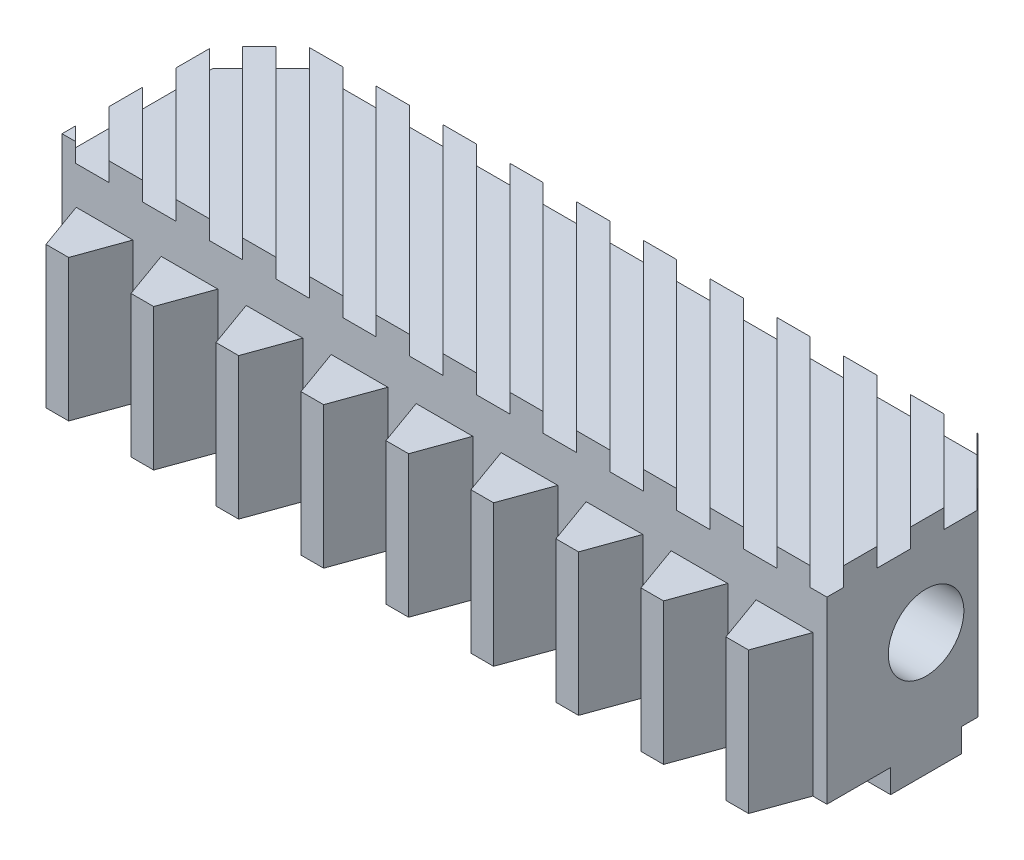
SolidWorks part; units mm, degrees
ref_plane "Front Plane" through (0, 0, 0) normal (0, 0, 1) x (1, 0, 0)
ref_plane "Top Plane" through (0, 0, 0) normal (0, 1, 0) x (1, 0, 0)
ref_plane "Right Plane" through (0, 0, 0) normal (1, 0, 0) x (0, 0, -1)
sketch "Sketch1" plane through (0, 0, 0) normal (0, 1, 0) x (1, 0, 0)
  line L0 (0, 0) -> (3.6, -10)
  line L1 (3.6, -10) -> (8.4, -10)
  line L2 (8.4, -10) -> (12, 0)
  line L3 (0, 0) -> (12, 0) construction
  line L4 (6, 0) -> (6, -10) construction
  line L5 (18, 0) -> (21.6, -10)
  line L6 (26.4, -10) -> (30, 0)
  line L7 (21.6, -10) -> (26.4, -10)
  line L8 (36, 0) -> (39.6, -10)
  line L9 (44.4, -10) -> (48, 0)
  line L10 (39.6, -10) -> (44.4, -10)
  line L11 (54, 0) -> (57.6, -10)
  line L12 (62.4, -10) -> (66, 0)
  line L13 (57.6, -10) -> (62.4, -10)
  line L14 (72, 0) -> (75.6, -10)
  line L15 (80.4, -10) -> (84, 0)
  line L16 (75.6, -10) -> (80.4, -10)
  line L17 (90, 0) -> (93.6, -10)
  line L18 (98.4, -10) -> (102, 0)
  line L19 (93.6, -10) -> (98.4, -10)
  line L20 (108, 0) -> (111.6, -10)
  line L21 (116.4, -10) -> (120, 0)
  line L22 (111.6, -10) -> (116.4, -10)
  line L23 (126, 0) -> (129.6, -10)
  line L24 (134.4, -10) -> (138, 0)
  line L25 (129.6, -10) -> (134.4, -10)
  line L26 (144, 0) -> (147.6, -10)
  line L27 (152.4, -10) -> (156, 0)
  line L28 (147.6, -10) -> (152.4, -10)
  line L29 (12, 0) -> (18, 0)
  line L30 (30, 0) -> (36, 0)
  line L31 (48, 0) -> (54, 0)
  line L32 (66, 0) -> (72, 0)
  line L33 (84, 0) -> (90, 0)
  line L34 (102, 0) -> (108, 0)
  line L35 (120, 0) -> (126, 0)
  line L36 (138, 0) -> (144, 0)
  line L37 (156, 0) -> (159, 0)
  line L38 (159, 0) -> (159, 42)
  line L39 (159, 42) -> (-3, 42)
  line L40 (-3, 42) -> (-3, 0)
  line L41 (-3, 0) -> (0, 0)
  dimension "D1" = 2.4
  dimension "D2" = 2.4
  dimension "D3" = 6
  dimension "D4" = 6
  dimension "D5" = 10
  dimension "D7" = 3
  dimension "D8" = 3
  dimension "D9" = 42
  dimension "D6" = 9
extrude "Boss-Extrude1" add sketch "Sketch1" along normal blind 30
sketch "Sketch2" plane through (0, 30, 0) normal (0, 1, 0) x (1, 0, 0)
  line L7 (26.4, -10) -> (39.6, -10)
  line L8 (39.6, -10) -> (36, 0)
  line L9 (-55, 0) -> (55, 0) construction
  line L10 (36, 0) -> (39.6, -10) construction
  line L11 (36, 0) -> (30, 0)
  line L12 (30, 0) -> (26.4, -10)
  line L13 (28.2, -5) -> (37.8, -5) construction
sketch "Sketch6" plane through (0, 30, 0) normal (0, 1, 0) x (1, 0, 0)
  line L0 (-16.5, 0) -> (16.5, 0) construction
  line L1 (-3, 42) -> (159, 42)
  line L2 (-3, 42) -> (-3, 0)
  line L3 (-3, 0) -> (159, 0)
  line L4 (159, 42) -> (159, 0)
  line L5 (159, 0) -> (159, 42) construction
extrude "Boss-Extrude2" add sketch "Sketch6" along normal blind 12
sketch "Sketch7" plane through (-3, 0, 0) normal (-1, 0, 0) x (0, 0, 1)
  line L0 (-42, 42) -> (0, 0) construction
  line L1 (-42, 0) -> (0, 0) construction
  circle A0 centre (-21, 21) radius 8
  dimension "D1" = 16
extrude "Cut-Extrude1" cut sketch "Sketch7" against normal through all both and the other way through all
sketch "Sketch9" plane through (-3, 0, 0) normal (-1, 0, 0) x (0, 0, 1)
  circle A0 centre (-21, 21) radius 8
  dimension "D1" = 16
sketch "Sketch10" plane through (0, 0, 0) normal (0, -1, 0) x (1, 0, 0)
  line L0 (-3, 0) -> (159, -42) construction
  line L1 (159, 0) -> (159, -42) construction
  line L2 (-3, -13.5) -> (159, -13.5)
  line L3 (-3, -13.5) -> (-3, -28.5)
  line L4 (-3, -28.5) -> (159, -28.5)
  line L5 (159, -13.5) -> (159, -28.5)
  line L6 (-3, -13.5) -> (159, -28.5) construction
  line L7 (-3, -28.5) -> (159, -13.5) construction
  point P4 (78, -21)
  dimension "D1" = 15
extrude "Boss-Extrude3" add sketch "Sketch10" along normal blind 5
sketch "Sketch12" plane through (0, 42, 0) normal (0, 1, 0) x (1, 0, 0)
  line L0 (40.6615, 118.3385) -> (159, 0) construction
  line L1 (17.5397, 141.4603) -> (40.6615, 118.3385) construction
  line L2 (159, 0) -> (196.8029, -37.8029) construction
  line L3 (48.5281, 110.4719) -> (221.9447, -62.9447) construction
  line L4 (50.2959, 112.2397) -> (223.7124, -61.1769)
  line L5 (46.7603, 108.7041) -> (220.1769, -64.7124)
  line L6 (135.2364, 23.7636) -> (142.7973, 31.3245) construction
  line L7 (159, 42) -> (-3, 42) construction
  line L8 (53.8314, 115.7752) -> (227.248, -57.6414)
  line L9 (57.3669, 119.3107) -> (230.7835, -54.1058)
  line L10 (55.5992, 117.543) -> (229.0157, -55.8736) construction
  line L11 (60.9025, 122.8463) -> (234.319, -50.5703)
  line L12 (64.438, 126.3818) -> (237.8546, -47.0348)
  line L13 (62.6702, 124.614) -> (236.0868, -48.8025) construction
  line L14 (67.9735, 129.9173) -> (241.3901, -43.4992)
  line L15 (71.5091, 133.4529) -> (244.9256, -39.9637)
  line L16 (69.7413, 131.6851) -> (243.1579, -41.7315) construction
  line L17 (39.6893, 101.6331) -> (213.1058, -71.7835)
  line L18 (43.2248, 105.1686) -> (216.6414, -68.248)
  line L19 (41.457, 103.4008) -> (214.8736, -70.0157) construction
  line L20 (32.6182, 94.562) -> (206.0348, -78.8546)
  line L21 (36.1537, 98.0975) -> (209.5703, -75.319)
  line L22 (34.386, 96.3298) -> (207.8025, -77.0868) construction
  line L23 (25.5471, 87.4909) -> (198.9637, -85.9256)
  line L24 (29.0827, 91.0265) -> (202.4992, -82.3901)
  line L25 (27.3149, 89.2587) -> (200.7315, -84.1579) construction
  line L26 (18.4761, 80.4199) -> (191.8926, -92.9967)
  line L27 (22.0116, 83.9554) -> (195.4282, -89.4612)
  line L28 (20.2438, 82.1876) -> (193.6604, -91.2289) construction
  line L29 (11.405, 73.3488) -> (184.8216, -100.0678)
  line L30 (14.9405, 76.8843) -> (188.3571, -96.5322)
  line L31 (13.1728, 75.1166) -> (186.5893, -98.3) construction
  line L32 (4.3339, 66.2777) -> (177.7505, -107.1388)
  line L33 (7.8695, 69.8133) -> (181.286, -103.6033)
  line L34 (6.1017, 68.0455) -> (179.5183, -105.3711) construction
  line L35 (-2.7372, 59.2067) -> (170.6794, -114.2099)
  line L36 (0.7984, 62.7422) -> (174.215, -110.6744)
  line L37 (-0.9694, 60.9744) -> (172.4472, -112.4421) construction
  line L38 (-9.8082, 52.1356) -> (163.6084, -121.281)
  line L39 (-6.2727, 55.6711) -> (167.1439, -117.7454)
  line L40 (-8.0405, 53.9034) -> (165.3761, -119.5132) construction
  line L41 (-16.8793, 45.0645) -> (156.5373, -128.352)
  line L42 (-13.3438, 48.6001) -> (160.0728, -124.8165)
  line L43 (-15.1115, 46.8323) -> (158.3051, -126.5843) construction
  line L44 (-23.9504, 37.9935) -> (149.4662, -135.4231)
  line L45 (-20.4148, 41.529) -> (153.0018, -131.8876)
  line L46 (-22.1826, 39.7612) -> (151.234, -133.6553) construction
  line L47 (-31.0214, 30.9224) -> (142.3951, -142.4942)
  line L48 (-27.4859, 34.4579) -> (145.9307, -138.9586)
  line L49 (-29.2537, 32.6902) -> (144.1629, -140.7264) construction
  line L50 (-38.0925, 23.8513) -> (135.3241, -149.5652)
  line L51 (-34.557, 27.3869) -> (138.8596, -146.0297)
  line L52 (-36.3247, 25.6191) -> (137.0918, -147.7975) construction
  arc A0 (50.2959, 112.2397) -> (46.7603, 108.7041) centre (48.5281, 110.4719) ccw
  arc A1 (220.1769, -64.7124) -> (223.7124, -61.1769) centre (221.9447, -62.9447) ccw
  arc A2 (57.3669, 119.3107) -> (53.8314, 115.7752) centre (55.5992, 117.543) ccw
  arc A3 (227.248, -57.6414) -> (230.7835, -54.1058) centre (229.0157, -55.8736) ccw
  arc A4 (64.438, 126.3818) -> (60.9025, 122.8463) centre (62.6702, 124.614) ccw
  arc A5 (234.319, -50.5703) -> (237.8546, -47.0348) centre (236.0868, -48.8025) ccw
  arc A6 (71.5091, 133.4529) -> (67.9735, 129.9173) centre (69.7413, 131.6851) ccw
  arc A7 (241.3901, -43.4992) -> (244.9256, -39.9637) centre (243.1579, -41.7315) ccw
  arc A8 (43.2248, 105.1686) -> (39.6893, 101.6331) centre (41.457, 103.4008) ccw
  arc A9 (213.1058, -71.7835) -> (216.6414, -68.248) centre (214.8736, -70.0157) ccw
  arc A10 (36.1537, 98.0975) -> (32.6182, 94.562) centre (34.386, 96.3298) ccw
  arc A11 (206.0348, -78.8546) -> (209.5703, -75.319) centre (207.8025, -77.0868) ccw
  arc A12 (29.0827, 91.0265) -> (25.5471, 87.4909) centre (27.3149, 89.2587) ccw
  arc A13 (198.9637, -85.9256) -> (202.4992, -82.3901) centre (200.7315, -84.1579) ccw
  arc A14 (22.0116, 83.9554) -> (18.4761, 80.4199) centre (20.2438, 82.1876) ccw
  arc A15 (191.8926, -92.9967) -> (195.4282, -89.4612) centre (193.6604, -91.2289) ccw
  arc A16 (14.9405, 76.8843) -> (11.405, 73.3488) centre (13.1728, 75.1166) ccw
  arc A17 (184.8216, -100.0678) -> (188.3571, -96.5322) centre (186.5893, -98.3) ccw
  arc A18 (7.8695, 69.8133) -> (4.3339, 66.2777) centre (6.1017, 68.0455) ccw
  arc A19 (177.7505, -107.1388) -> (181.286, -103.6033) centre (179.5183, -105.3711) ccw
  arc A20 (0.7984, 62.7422) -> (-2.7372, 59.2067) centre (-0.9694, 60.9744) ccw
  arc A21 (170.6794, -114.2099) -> (174.215, -110.6744) centre (172.4472, -112.4421) ccw
  arc A22 (-6.2727, 55.6711) -> (-9.8082, 52.1356) centre (-8.0405, 53.9034) ccw
  arc A23 (163.6084, -121.281) -> (167.1439, -117.7454) centre (165.3761, -119.5132) ccw
  arc A24 (-13.3438, 48.6001) -> (-16.8793, 45.0645) centre (-15.1115, 46.8323) ccw
  arc A25 (156.5373, -128.352) -> (160.0728, -124.8165) centre (158.3051, -126.5843) ccw
  arc A26 (-20.4148, 41.529) -> (-23.9504, 37.9935) centre (-22.1826, 39.7612) ccw
  arc A27 (149.4662, -135.4231) -> (153.0018, -131.8876) centre (151.234, -133.6553) ccw
  arc A28 (-27.4859, 34.4579) -> (-31.0214, 30.9224) centre (-29.2537, 32.6902) ccw
  arc A29 (142.3951, -142.4942) -> (145.9307, -138.9586) centre (144.1629, -140.7264) ccw
  arc A30 (-34.557, 27.3869) -> (-38.0925, 23.8513) centre (-36.3247, 25.6191) ccw
  arc A31 (135.3241, -149.5652) -> (138.8596, -146.0297) centre (137.0918, -147.7975) ccw
  point P8 (135.2364, 23.7636)
  point P20 (142.3074, 30.8347)
  point P27 (149.3785, 37.9058)
  point P34 (156.4496, 44.9768)
  point P41 (128.1653, 16.6926)
  point P48 (121.0942, 9.6215)
  point P55 (114.0232, 2.5504)
  point P62 (106.9521, -4.5206)
  point P69 (99.881, -11.5917)
  point P76 (92.81, -18.6628)
  point P83 (85.7389, -25.7339)
  point P90 (78.6678, -32.8049)
  point P97 (71.5968, -39.876)
  point P104 (64.5257, -46.9471)
  point P111 (57.4546, -54.0181)
  point P118 (50.3836, -61.0892)
  dimension "D1" = 5
  dimension "D2" = 45
  dimension "D3" = 4
  dimension "D4" = 13
extrude "Cut-Extrude3" cut sketch "Sketch12" against normal blind 4
sketch "Sketch13" plane through (0, 42, 0) normal (0, 1, 0) x (1, 0, 0)
  line L0 (93.21, 69.3256) -> (60.6108, 36.7264)
  line L1 (159, 3.5355) -> (120.5355, 42) construction
  line L2 (159, 3.5355) -> (120.5355, 42) construction
chamfer "Chamfer1" distance 10 angle 45 2 edges at (-3, 21, -42) (159, 19, -42)
